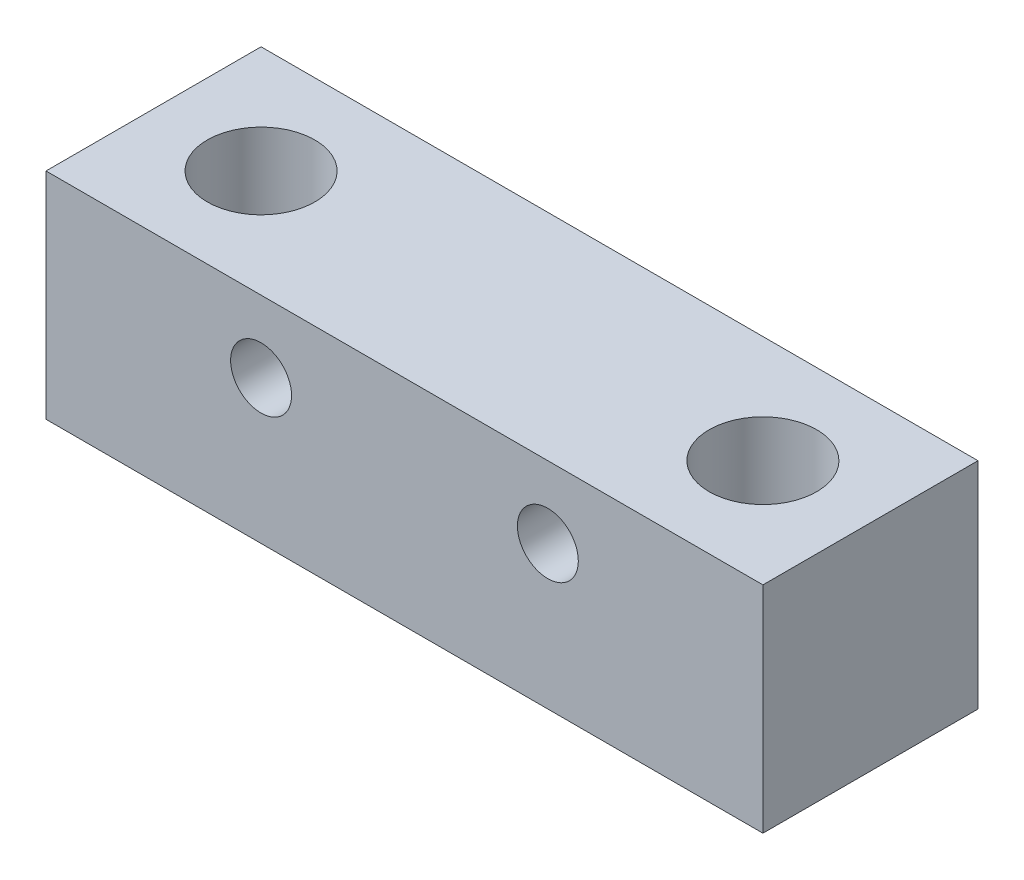
from build123d import *

# Parameters (mm, degrees)
SKETCH_1_W                = 100
SKETCH_1_H                = 30
EXTRUDE_1_DEPTH           = 30
HOLE_WIZARD_1_D           = 9
HOLE_WIZARD_1_CBORE_D     = 15
HOLE_WIZARD_1_CBORE_DEPTH = 20
HOLE_WIZARD_M10_1_D       = 8.5


with BuildPart() as part:
    # 草图1 → 凸台-拉伸1 (new body)
    with BuildSketch(Plane.XY):
        Rectangle(SKETCH_1_W, SKETCH_1_H)
    extrude(amount=EXTRUDE_1_DEPTH)

    # 打孔尺寸(%根据)内六角圆柱头螺钉的类型1 (through all)
    with Locations(Plane(origin=(0, 15, 0), x_dir=(1, 0, 0), z_dir=(0, 1, 0))):
        with Locations((-35, -15), (35, -15)):
            CounterBoreHole(HOLE_WIZARD_1_D / 2, HOLE_WIZARD_1_CBORE_D / 2, HOLE_WIZARD_1_CBORE_DEPTH)

    # M10 螺纹孔1 (through all)
    with Locations(Plane.XY.offset(30)):
        with Locations((-20, 5), (20, 5)):
            Hole(HOLE_WIZARD_M10_1_D / 2)


solid = part.part
